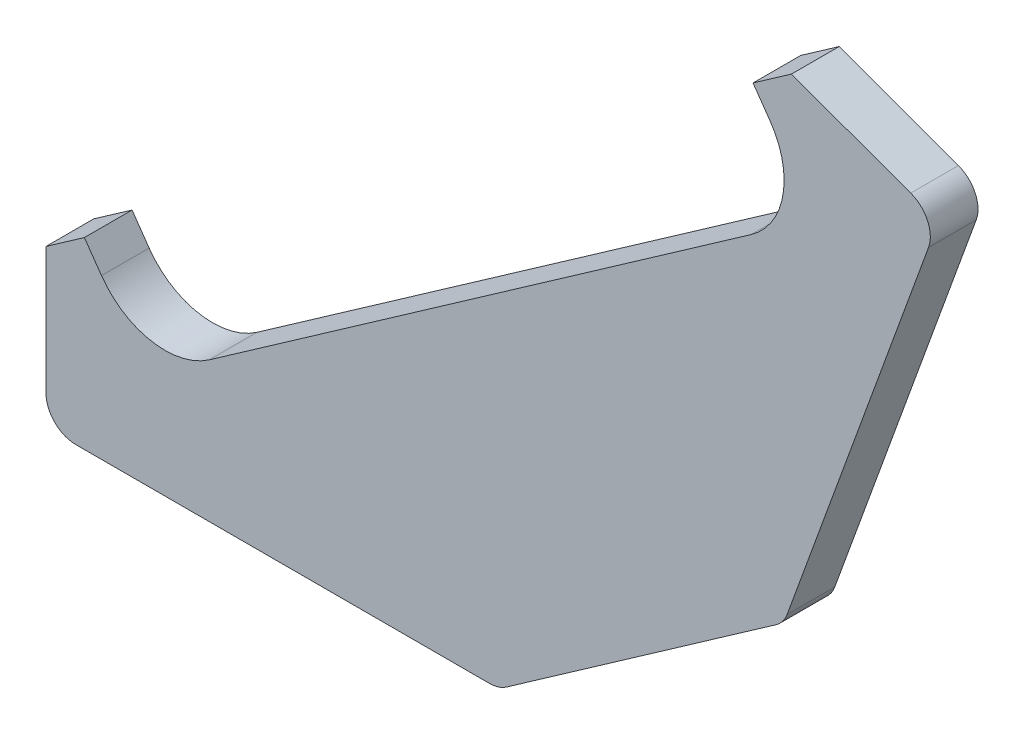
from build123d import *

# Parameters (mm, degrees)
EXTRUDE_1_DEPTH = 16
FILLET_1_R      = 10


with BuildPart() as part:
    # 草图1 → 凸台-拉伸1 (new body)
    with BuildSketch(Plane.XY):
        with BuildLine():
            Line((-132, 141.901665764), (-152, 141.901665764))
            Line((-152, 141.901665764), (-152, 194.51841477))
            Line((-152, 194.51841477), (-139.107955396, 203.545521584))
            Line((-139.107955396, 203.545521584), (-133.372191032, 195.354001142))
            ThreePointArc((-133.372191032, 195.354001142), (-116.5890905, 184.661986908), (-97.161250536, 188.969035335))
            Line((-97.161250536, 188.969035335), (84.690503297, 316.303004205))
            ThreePointArc((84.690503297, 316.303004205), (95.38251753, 333.086104737), (91.075469103, 352.513944702))
            Line((91.075469103, 352.513944702), (85.339704739, 360.705465145))
            Line((85.339704739, 360.705465145), (98.231749344, 369.732571959))
            Line((98.231749344, 369.732571959), (147.675320114, 351.736583923))
            Line((147.675320114, 351.736583923), (140.834917247, 332.942731507))
            Line((140.834917247, 332.942731507), (95.688258328, 208.903305564))
            Line((95.688258328, 208.903305564), (0, 141.901665764))
            Line((0, 141.901665764), (-132, 141.901665764))
        make_face()
    extrude(amount=EXTRUDE_1_DEPTH)

    # 圆角1
    fillet_1_edges = [part.edges().sort_by_distance(p)[0] for p in [
        (-152, 141.901665764, 8),
        (147.675320114, 351.736583923, 8),
        (95.688258328, 208.903305564, 8),
        (0, 141.901665764, 8),
    ]]
    fillet(fillet_1_edges, radius=FILLET_1_R)


solid = part.part
